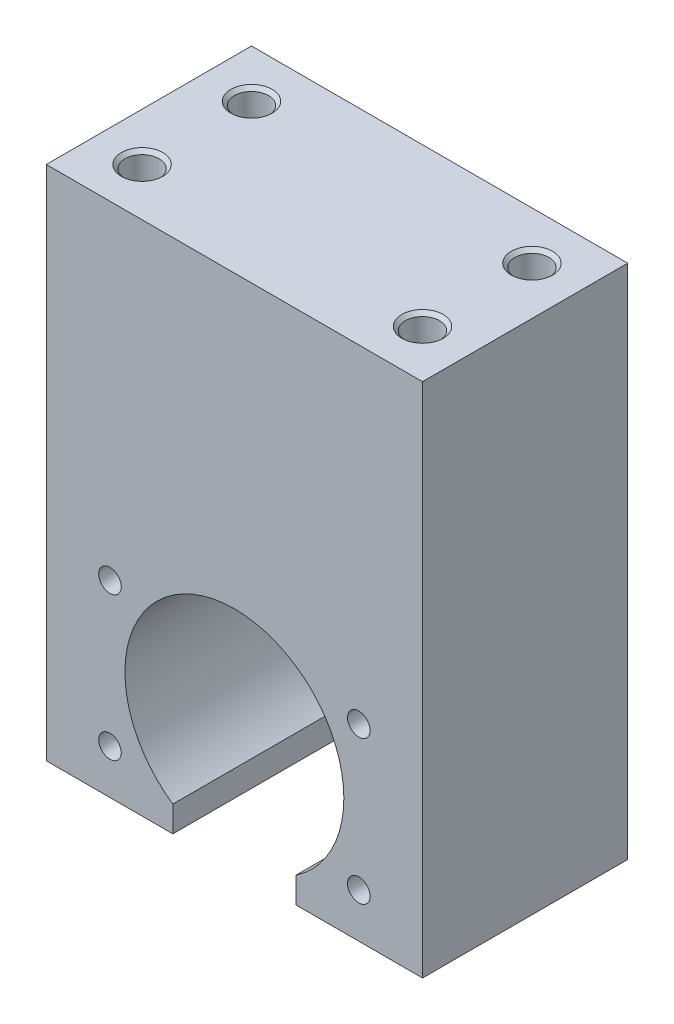
from build123d import *

# Parameters (mm, degrees)
EXTRUDE_1_DEPTH              = 15
HOLE_WIZARD_M4_1_D           = 3.3
HOLE_WIZARD_M4_1_DEPTH       = 9.5
HOLE_WIZARD_M4_1_TIP         = 0.991420021
HOLE_WIZARD_M6_1_D           = 5
HOLE_WIZARD_M6_1_DEPTH       = 12
HOLE_WIZARD_M6_1_CSINK_D     = 6.05
HOLE_WIZARD_M6_1_CSINK_ANGLE = 90
HOLE_WIZARD_M6_1_TIP         = 1.502151548


with BuildPart() as part:
    # 草图1 → 凸台-拉伸1 (new, symmetric)
    with BuildSketch(Plane.XY):
        with BuildLine():
            Line((-27.5, 58.5), (27.5, 58.5))
            Line((27.5, 58.5), (27.5, -17))
            Line((27.5, -17), (9, -17))
            Line((9, -17), (9, -13.228756555))
            ThreePointArc((9, -13.228756555), (0, 16), (-9, -13.228756555))
            Line((-9, -13.228756555), (-9, -17))
            Line((-9, -17), (-27.5, -17))
            Line((-27.5, -17), (-27.5, 58.5))
        make_face()
    extrude(amount=EXTRUDE_1_DEPTH, both=True)

    # M4 螺纹孔1
    with Locations(Plane.XY.offset(15)):
        with Locations((18.186533479, 10.5), (18.186533479, -10.5), (-18.186533479, -10.5), (-18.186533479, 10.5)):
            Hole(HOLE_WIZARD_M4_1_D / 2, depth=HOLE_WIZARD_M4_1_DEPTH)
            with Locations((0, 0, -(HOLE_WIZARD_M4_1_DEPTH + HOLE_WIZARD_M4_1_TIP / 2))):  # 118° drill point
                Cone(0, HOLE_WIZARD_M4_1_D / 2, HOLE_WIZARD_M4_1_TIP, mode=Mode.SUBTRACT)

    # M6 螺纹孔1
    with Locations(Plane(origin=(-20.5, 58.5, 8), x_dir=(0, 0, 1), z_dir=(0, 1, 0))):
        with Locations((0, 0), (-16, 0), (-16, 41), (0, 41)):
            CounterSinkHole(HOLE_WIZARD_M6_1_D / 2, HOLE_WIZARD_M6_1_CSINK_D / 2, depth=HOLE_WIZARD_M6_1_DEPTH, counter_sink_angle=HOLE_WIZARD_M6_1_CSINK_ANGLE)
            with Locations((0, 0, -(HOLE_WIZARD_M6_1_DEPTH + HOLE_WIZARD_M6_1_TIP / 2))):  # 118° drill point
                Cone(0, HOLE_WIZARD_M6_1_D / 2, HOLE_WIZARD_M6_1_TIP, mode=Mode.SUBTRACT)


solid = part.part
